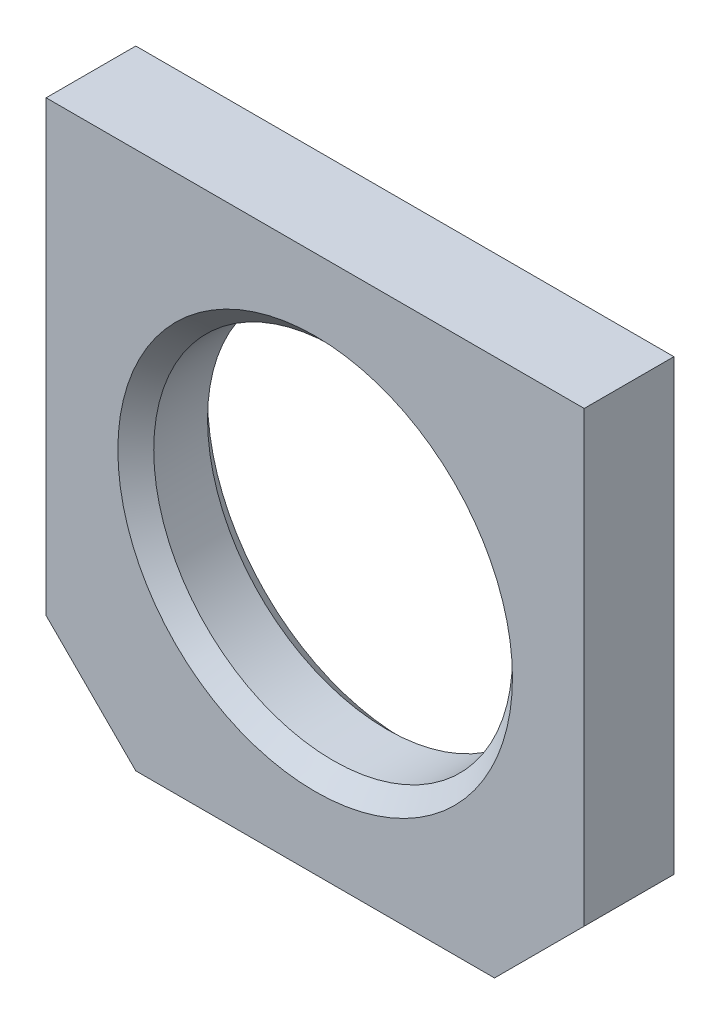
SolidWorks part; units mm, degrees
material "Q235-A"
ref_plane "前视基准面" through (0, 0, 0) normal (0, 0, 1) x (1, 0, 0)
ref_plane "上视基准面" through (0, 0, 0) normal (0, 1, 0) x (1, 0, 0)
ref_plane "右视基准面" through (0, 0, 0) normal (1, 0, 0) x (0, 0, -1)
sketch "草图1" plane through (0, 0, 0) normal (0, 0, 1) x (1, 0, 0)
  line L1 (-30, -30) -> (30, -30)
  line L2 (-30, -30) -> (-30, 30)
  line L3 (-30, 30) -> (30, 30)
  line L4 (30, -30) -> (30, 30)
  line L5 (-30, -30) -> (30, 30) construction
  line L6 (-30, 30) -> (30, -30) construction
  circle A0 centre (0, 0) radius 20
  point P0 (0, 0)
  dimension "D3" = 40
  dimension "D1" = 60
  dimension "D2" = 60
extrude "凸台-拉伸1" add sketch "草图1" along normal blind 10
chamfer "倒角1" distance 10 angle 45 2 edges at (30, -30, 5) (-30, -30, 5)
chamfer "倒角3" distance 2 angle 45 2 edges at (20, 0, 0) (20, 0, 10)
